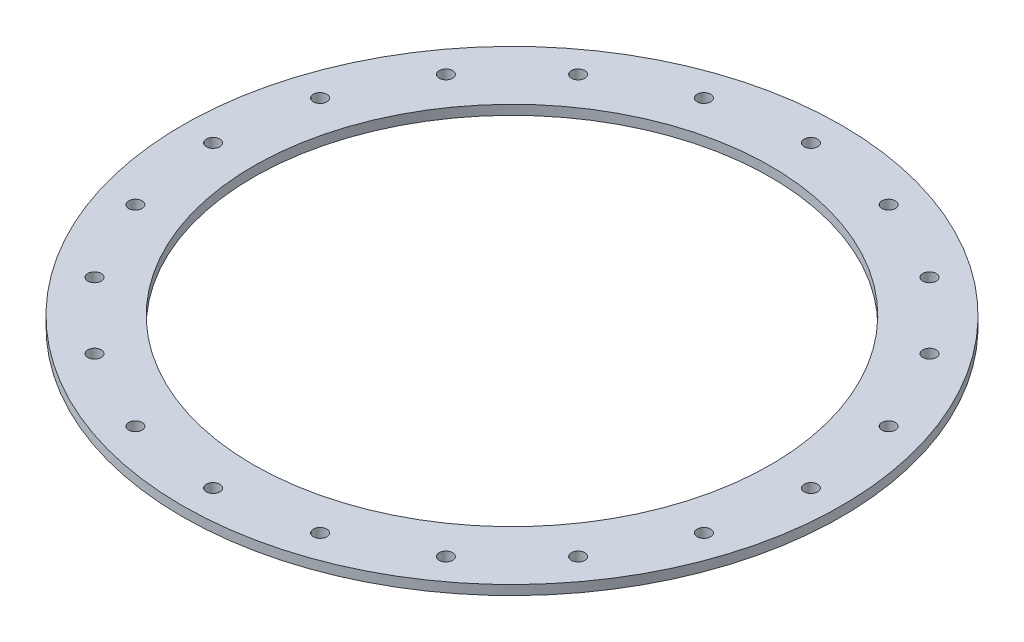
SolidWorks part; units mm, degrees
material "Q235B"
ref_plane "前视基准面" through (0, 0, 0) normal (0, 0, 1) x (1, 0, 0)
ref_plane "上视基准面" through (0, 0, 0) normal (0, 1, 0) x (1, 0, 0)
ref_plane "右视基准面" through (0, 0, 0) normal (1, 0, 0) x (0, 0, -1)
sketch "草图1" plane through (0, 0, 0) normal (0, 1, 0) x (1, 0, 0)
  circle A0 centre (0, 0) radius 675
  circle A1 centre (0, 0) radius 860
  dimension "D1" = 1350
  dimension "D2" = 1720
extrude "凸台-拉伸1" add sketch "草图1" along normal blind 25
hole_wizard "Ø25.5 (25.5) 直径孔1" positions "草图3" profile "草图4" hole size "Ø25.5" standard "GB" end condition up to next
sketch "草图3" plane through (0, 25, 0) normal (0, 1, 0) x (1, 0, 0)
  line L0 (0, 0) -> (0, 780) construction
  circle A1 centre (0, 0) radius 780
  point P0 (0, 780)
  point P16 (241.0333, 741.8241)
  point P17 (458.4725, 631.0333)
  point P18 (631.0333, 458.4725)
  point P19 (741.8241, 241.0333)
  point P20 (780, 0)
  point P21 (741.8241, -241.0333)
  point P22 (631.0333, -458.4725)
  point P23 (458.4725, -631.0333)
  point P24 (241.0333, -741.8241)
  point P25 (0, -780)
  point P26 (-241.0333, -741.8241)
  point P27 (-458.4725, -631.0333)
  point P28 (-631.0333, -458.4725)
  point P29 (-741.8241, -241.0333)
  point P30 (-780, 0)
  point P31 (-741.8241, 241.0333)
  point P32 (-631.0333, 458.4725)
  point P33 (-458.4725, 631.0333)
  point P34 (-241.0333, 741.8241)
  dimension "D1" = 1560
  dimension "D2" = 20
sketch "草图4" plane through (0, 25, -780) normal (1, 0, 0) x (0, 0, 1)
  line L0 (0, 0) -> (0, 25)
  line L1 (0, 25) -> (17.5, 25)
  line L2 (17.5, 25) -> (17.5, 0)
  line L5 (17.5, 0) -> (0, 0)
  line L11 (0, -6.35) -> (0, 107.95) construction
  dimension "通孔孔直径" = 35
  dimension "通孔孔深度" = 25
